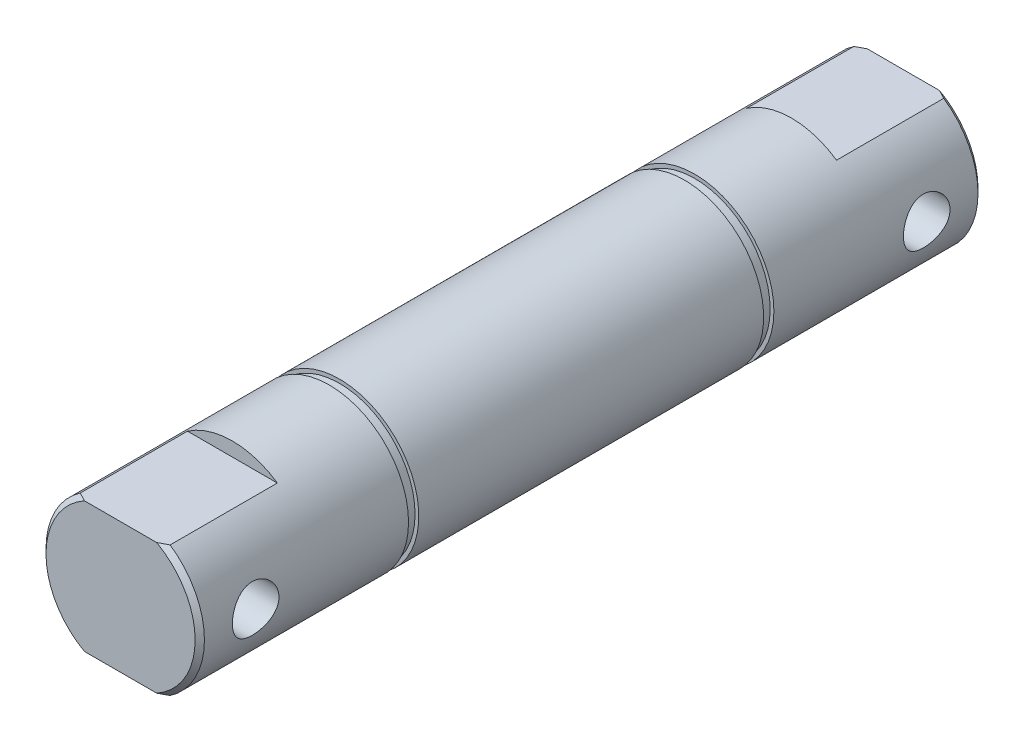
from build123d import *

# Parameters (mm, degrees)
SKETCH_1_R          = 8.5
EXTRUDE_1_DEPTH     = 42
SKETCH_2_W          = 25
SKETCH_2_H          = 3
CUT_EXTRUDE_1_DEPTH = 12
CHAMFER_2_SIZE      = 0.5
HOLE_WIZARD_M6_1_D  = 5
SKETCH_5_W          = 0.4
SKETCH_5_H          = 1.1


with BuildPart() as part:
    # 草图1 → 凸台-拉伸1 (new, symmetric)
    with BuildSketch(Plane.XY):
        with Locations(Location((0, 0, 0), (0, 0, 180))):
            Circle(SKETCH_1_R)
    extrude(amount=EXTRUDE_1_DEPTH, both=True)

    # 草图2 → 切除-拉伸1 (cut)
    with BuildSketch(Plane.XY.offset(42)):
        with Locations((0, 8.5)):
            Rectangle(SKETCH_2_W, SKETCH_2_H)
        with Locations((0, -8.5)):
            Rectangle(SKETCH_2_W, SKETCH_2_H)
    cut_extrude_1 = extrude(amount=-CUT_EXTRUDE_1_DEPTH, mode=Mode.SUBTRACT)

    # 镜向1: 切除-拉伸1 across plane
    add(cut_extrude_1.mirror(Plane.XY), mode=Mode.SUBTRACT)

    # 倒角2
    chamfer_2_edges = [part.edges().sort_by_distance(p)[0] for p in [
        (8.5, 0, 42),
        (-7.524477249, 3.953763034, -42),
        (8.5, 0, -42),
        (-7.524477249, 3.953763034, 42),
    ]]
    chamfer(chamfer_2_edges, length=CHAMFER_2_SIZE)

    # M6 螺纹孔1 (through all)
    with Locations(Plane(origin=(8.5, 0, 0), x_dir=(0, 0, -1), z_dir=(1, 0, 0))):
        with Locations((-36, 0), (36, 0)):
            Hole(HOLE_WIZARD_M6_1_D / 2)

    # 草图5 → 切除-旋转1 (revolve, cut)
    with BuildSketch(Plane(origin=(0, 0, 0), x_dir=(1, 0, 0), z_dir=(0, 1, 0)), mode=Mode.PRIVATE) as cut_revolve_1_sk:
        with Locations((-8.3, 19.05)):
            Rectangle(SKETCH_5_W, SKETCH_5_H)
        with Locations((-8.3, -19.05)):
            Rectangle(SKETCH_5_W, SKETCH_5_H)
    revolve(cut_revolve_1_sk.sketch.rotate(Axis((0, 0, 0), (0, 0, -1)), 180), axis=Axis((0, 0, 0), (0, 0, -1)), mode=Mode.SUBTRACT)


solid = part.part
